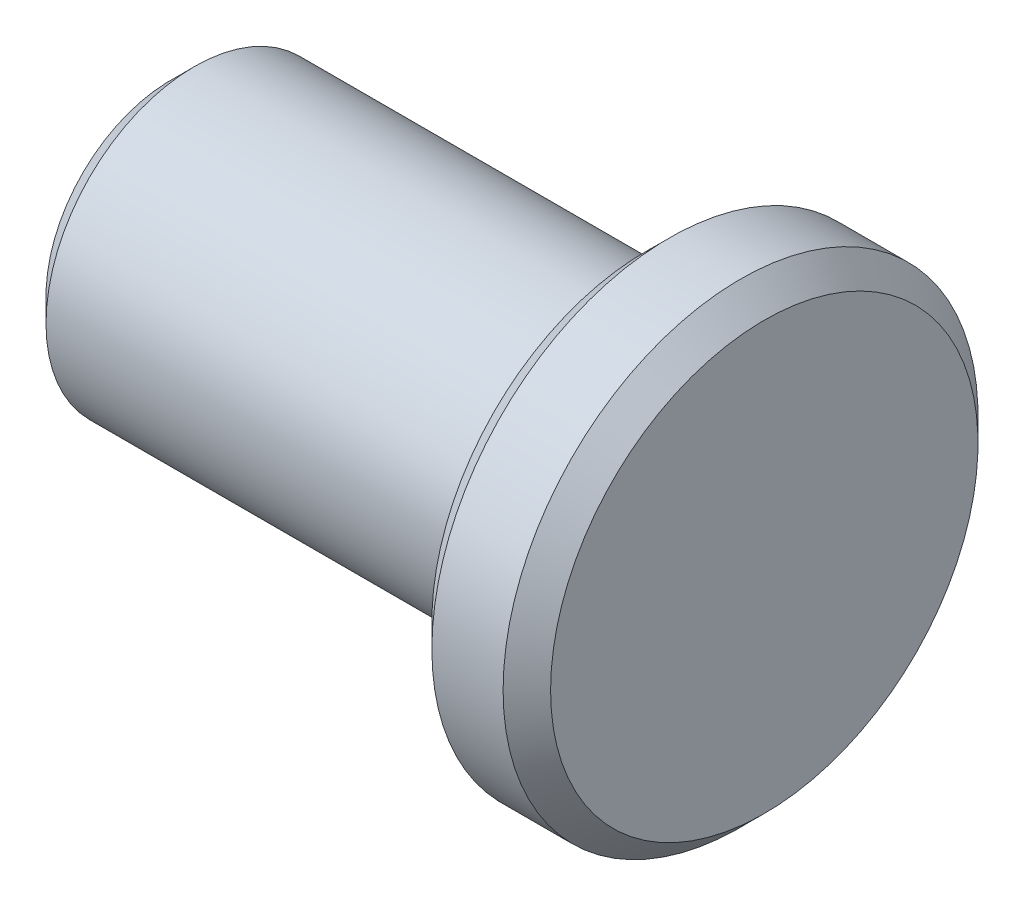
from build123d import *

# Parameters (mm, degrees)
CHAMFER_1_SIZE = 1


with BuildPart() as part:
    # 草图1 → 旋转1 (revolve)
    with BuildSketch(Plane.XY, mode=Mode.PRIVATE) as revolve_1_sk:
        Polygon((236.937142185, -170.509032878), (236.937142185, -164.259032878), (256.937142185, -164.259032878), (256.937142185, -160.509032878), (261.937142185, -160.509032878), (261.937142185, -170.509032878), align=None)
    revolve(revolve_1_sk.sketch.rotate(Axis((232.937142185, -170.509032878, 0), (1, 0, 0)), 90), axis=Axis((232.937142185, -170.509032878, 0), (1, 0, 0)))

    # 倒角1
    chamfer_1_edges = [part.edges().sort_by_distance(p)[0] for p in [
        (261.937142185, -170.509032878, -10),
        (256.937142185, -170.509032878, -10),
        (236.937142185, -170.509032878, -6.25),
    ]]
    chamfer(chamfer_1_edges, length=CHAMFER_1_SIZE)


solid = part.part
